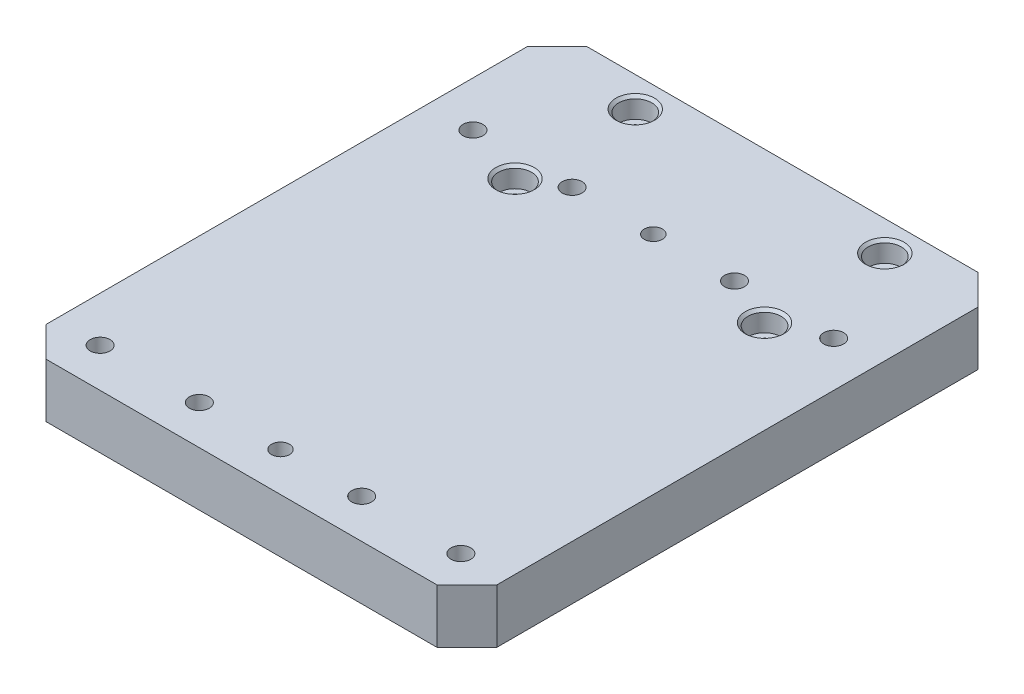
from build123d import *

# Parameters (mm, degrees)
SKETCH_1_W               = 150
SKETCH_1_H               = 180
EXTRUDE_1_DEPTH          = 18
CHAMFER_1_SIZE           = 10
HOLE_WIZARD_1_AT_2_COUNT = 2
HOLE_WIZARD_1_AT_2_PITCH = 33
HOLE_WIZARD_1_AT_3_COUNT = 2
HOLE_WIZARD_1_AT_3_PITCH = 87
HOLE_WIZARD_1_AT_4_COUNT = 2
HOLE_WIZARD_1_AT_4_PITCH = 120
HOLE_WIZARD_1_AT_5_COUNT = 2
HOLE_WIZARD_1_AT_5_PITCH = 124
HOLE_WIZARD_1_AT_6_COUNT = 2
HOLE_WIZARD_1_AT_6_PITCH = 128.316016148
HOLE_WIZARD_1_AT_7_COUNT = 2
HOLE_WIZARD_1_AT_7_PITCH = 151.476070717
HOLE_WIZARD_1_AT_8_COUNT = 2
HOLE_WIZARD_1_AT_8_PITCH = 172.557236881
SKETCH_6_R               = 3
CUT_EXTRUDE_1_DEPTH      = 119.528477591
HOLE_WIZARD_2_AT_2_COUNT = 2
HOLE_WIZARD_2_AT_2_PITCH = 40
HOLE_WIZARD_2_AT_3_COUNT = 2
HOLE_WIZARD_2_AT_3_PITCH = 92.135769384
HOLE_WIZARD_2_AT_4_COUNT = 2
HOLE_WIZARD_2_AT_4_PITCH = 83


with BuildPart() as part:
    # 草图1 → 凸台-拉伸1 (new body)
    with BuildSketch(Plane(origin=(0, 0, 0), x_dir=(1, 0, 0), z_dir=(0, 1, 0))):
        Rectangle(SKETCH_1_W, SKETCH_1_H)
    extrude(amount=EXTRUDE_1_DEPTH)

    # 倒角1
    chamfer_1_edges = [part.edges().sort_by_distance(p)[0] for p in [
        (75, 9, 90),
        (-75, 9, 90),
        (-75, 9, -90),
        (75, 9, -90),
    ]]
    chamfer(chamfer_1_edges, length=CHAMFER_1_SIZE)

    # 草图5 → 打孔尺寸(%根据)内六角圆柱头螺钉的类型1 (revolve, cut)
    with BuildSketch(Plane(origin=(60, 0, -46.999999026), x_dir=(0, 0, -1), z_dir=(1, 0, 0))):
        Polygon((0, 0), (0, 18), (3.3, 18), (3.3, 6.8), (5.5, 6.8), (5.5, 1.025), (6.525, 0), align=None)
    hole_wizard_1 = revolve(axis=Axis((60, -6.35, -46.999999026), (0, 1, 0)), mode=Mode.SUBTRACT)

    # 打孔尺寸(%根据)内六角圆柱头螺钉的类型1 at 2: 打孔尺寸(%根据)内六角圆柱头螺钉的类型1 ×2
    with Locations(*[(-i * HOLE_WIZARD_1_AT_2_PITCH, 0, 0) for i in range(1, HOLE_WIZARD_1_AT_2_COUNT)]):
        add(hole_wizard_1, mode=Mode.SUBTRACT)

    # 打孔尺寸(%根据)内六角圆柱头螺钉的类型1 at 3: 打孔尺寸(%根据)内六角圆柱头螺钉的类型1 ×2
    with Locations(*[(-i * HOLE_WIZARD_1_AT_3_PITCH, 0, 0) for i in range(1, HOLE_WIZARD_1_AT_3_COUNT)]):
        add(hole_wizard_1, mode=Mode.SUBTRACT)

    # 打孔尺寸(%根据)内六角圆柱头螺钉的类型1 at 4: 打孔尺寸(%根据)内六角圆柱头螺钉的类型1 ×2
    with Locations(*[(-i * HOLE_WIZARD_1_AT_4_PITCH, 0, 0) for i in range(1, HOLE_WIZARD_1_AT_4_COUNT)]):
        add(hole_wizard_1, mode=Mode.SUBTRACT)

    # 打孔尺寸(%根据)内六角圆柱头螺钉的类型1 at 5: 打孔尺寸(%根据)内六角圆柱头螺钉的类型1 ×2
    with Locations(*[(0, 0, i * HOLE_WIZARD_1_AT_5_PITCH) for i in range(1, HOLE_WIZARD_1_AT_5_COUNT)]):
        add(hole_wizard_1, mode=Mode.SUBTRACT)

    # 打孔尺寸(%根据)内六角圆柱头螺钉的类型1 at 6: 打孔尺寸(%根据)内六角圆柱头螺钉的类型1 ×2
    with Locations(*[Vector(-0.25717756045339407, 0, 0.9663641665538105) * (i * HOLE_WIZARD_1_AT_6_PITCH) for i in range(1, HOLE_WIZARD_1_AT_6_COUNT)]):
        add(hole_wizard_1, mode=Mode.SUBTRACT)

    # 打孔尺寸(%根据)内六角圆柱头螺钉的类型1 at 7: 打孔尺寸(%根据)内六角圆柱头螺钉的类型1 ×2
    with Locations(*[Vector(-0.5743481434915226, 0, 0.8186111470459227) * (i * HOLE_WIZARD_1_AT_7_PITCH) for i in range(1, HOLE_WIZARD_1_AT_7_COUNT)]):
        add(hole_wizard_1, mode=Mode.SUBTRACT)

    # 打孔尺寸(%根据)内六角圆柱头螺钉的类型1 at 8: 打孔尺寸(%根据)内六角圆柱头螺钉的类型1 ×2
    with Locations(*[Vector(-0.6954214275158859, 0, 0.7186021417667552) * (i * HOLE_WIZARD_1_AT_8_PITCH) for i in range(1, HOLE_WIZARD_1_AT_8_COUNT)]):
        add(hole_wizard_1, mode=Mode.SUBTRACT)

    # 草图6 → 切除-拉伸1 (cut, through all)
    with BuildSketch(Plane.XZ):
        with Locations(Location((0, -46.999999026, 0), (0, 0, 270))):
            Circle(SKETCH_6_R)
        with Locations(Location((0, 77.000000974, 0), (0, 0, 270))):
            Circle(SKETCH_6_R)
    extrude(amount=-CUT_EXTRUDE_1_DEPTH, mode=Mode.SUBTRACT)

    # 草图8 → 打孔尺寸(%根据)内六角圆柱头螺钉的类型2 (revolve, cut)
    with BuildSketch(Plane(origin=(-39, 18, -40), x_dir=(0, 0, 1), z_dir=(1, 0, 0))):
        Polygon((0, 0), (0, 18), (3.3, 18), (3.3, 6.8), (5.5, 6.8), (5.5, 0.9), (6.4, 0), align=None)
    hole_wizard_2 = revolve(axis=Axis((-39, 24.35, -40), (0, -1, 0)), mode=Mode.SUBTRACT)

    # 打孔尺寸(%根据)内六角圆柱头螺钉的类型2 at 2: 打孔尺寸(%根据)内六角圆柱头螺钉的类型2 ×2
    with Locations(*[(0, 0, -i * HOLE_WIZARD_2_AT_2_PITCH) for i in range(1, HOLE_WIZARD_2_AT_2_COUNT)]):
        add(hole_wizard_2, mode=Mode.SUBTRACT)

    # 打孔尺寸(%根据)内六角圆柱头螺钉的类型2 at 3: 打孔尺寸(%根据)内六角圆柱头螺钉的类型2 ×2
    with Locations(*[Vector(0.9008444880292467, 0, -0.4341419219418052) * (i * HOLE_WIZARD_2_AT_3_PITCH) for i in range(1, HOLE_WIZARD_2_AT_3_COUNT)]):
        add(hole_wizard_2, mode=Mode.SUBTRACT)

    # 打孔尺寸(%根据)内六角圆柱头螺钉的类型2 at 4: 打孔尺寸(%根据)内六角圆柱头螺钉的类型2 ×2
    with Locations(*[(i * HOLE_WIZARD_2_AT_4_PITCH, 0, 0) for i in range(1, HOLE_WIZARD_2_AT_4_COUNT)]):
        add(hole_wizard_2, mode=Mode.SUBTRACT)


solid = part.part
